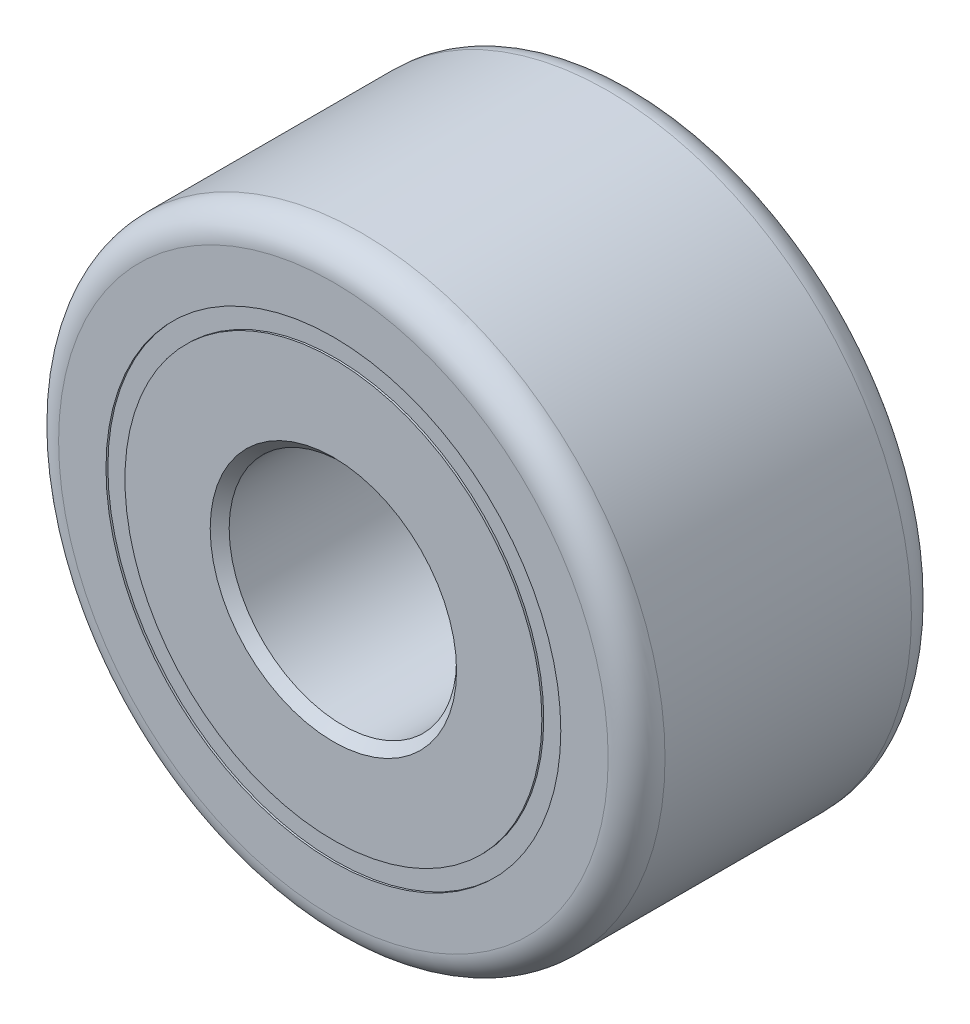
from build123d import *

# Parameters (mm, degrees)
SKETCH1_R           = 16
BOSS_EXTRUDE1_DEPTH = 16
SKETCH2_R           = 6
CUT_EXTRUDE1_DEPTH  = 16
SKETCH3_R           = 12
SKETCH3_R_2         = 11
CUT_EXTRUDE2_DEPTH  = 0.1
FILLET1_R           = 1.5
CHAMFER1_SIZE       = 0.5


with BuildPart() as part:
    # Sketch1 → Boss-Extrude1 (new body)
    with BuildSketch(Plane.XY):
        Circle(SKETCH1_R)
    extrude(amount=BOSS_EXTRUDE1_DEPTH)

    # Sketch2 → Cut-Extrude1 (cut)
    with BuildSketch(Plane.XY.offset(16)):
        Circle(SKETCH2_R)
    extrude(amount=-CUT_EXTRUDE1_DEPTH, mode=Mode.SUBTRACT)

    # Sketch3 → Cut-Extrude2 (cut)
    with BuildSketch(Plane.XY.offset(16)):
        Circle(SKETCH3_R)
        Circle(SKETCH3_R_2, mode=Mode.SUBTRACT)
    extrude(amount=-CUT_EXTRUDE2_DEPTH, mode=Mode.SUBTRACT)

    # Fillet1
    fillet1_edges = [part.edges().sort_by_distance(p)[0] for p in [
        (-16, 0, 0),
        (-16, 0, 16),
    ]]
    fillet(fillet1_edges, radius=FILLET1_R)

    # Chamfer1
    chamfer1_edges = [part.edges().sort_by_distance(p)[0] for p in [
        (-6, 0, 0),
        (-6, 0, 16),
    ]]
    chamfer(chamfer1_edges, length=CHAMFER1_SIZE)


solid = part.part
